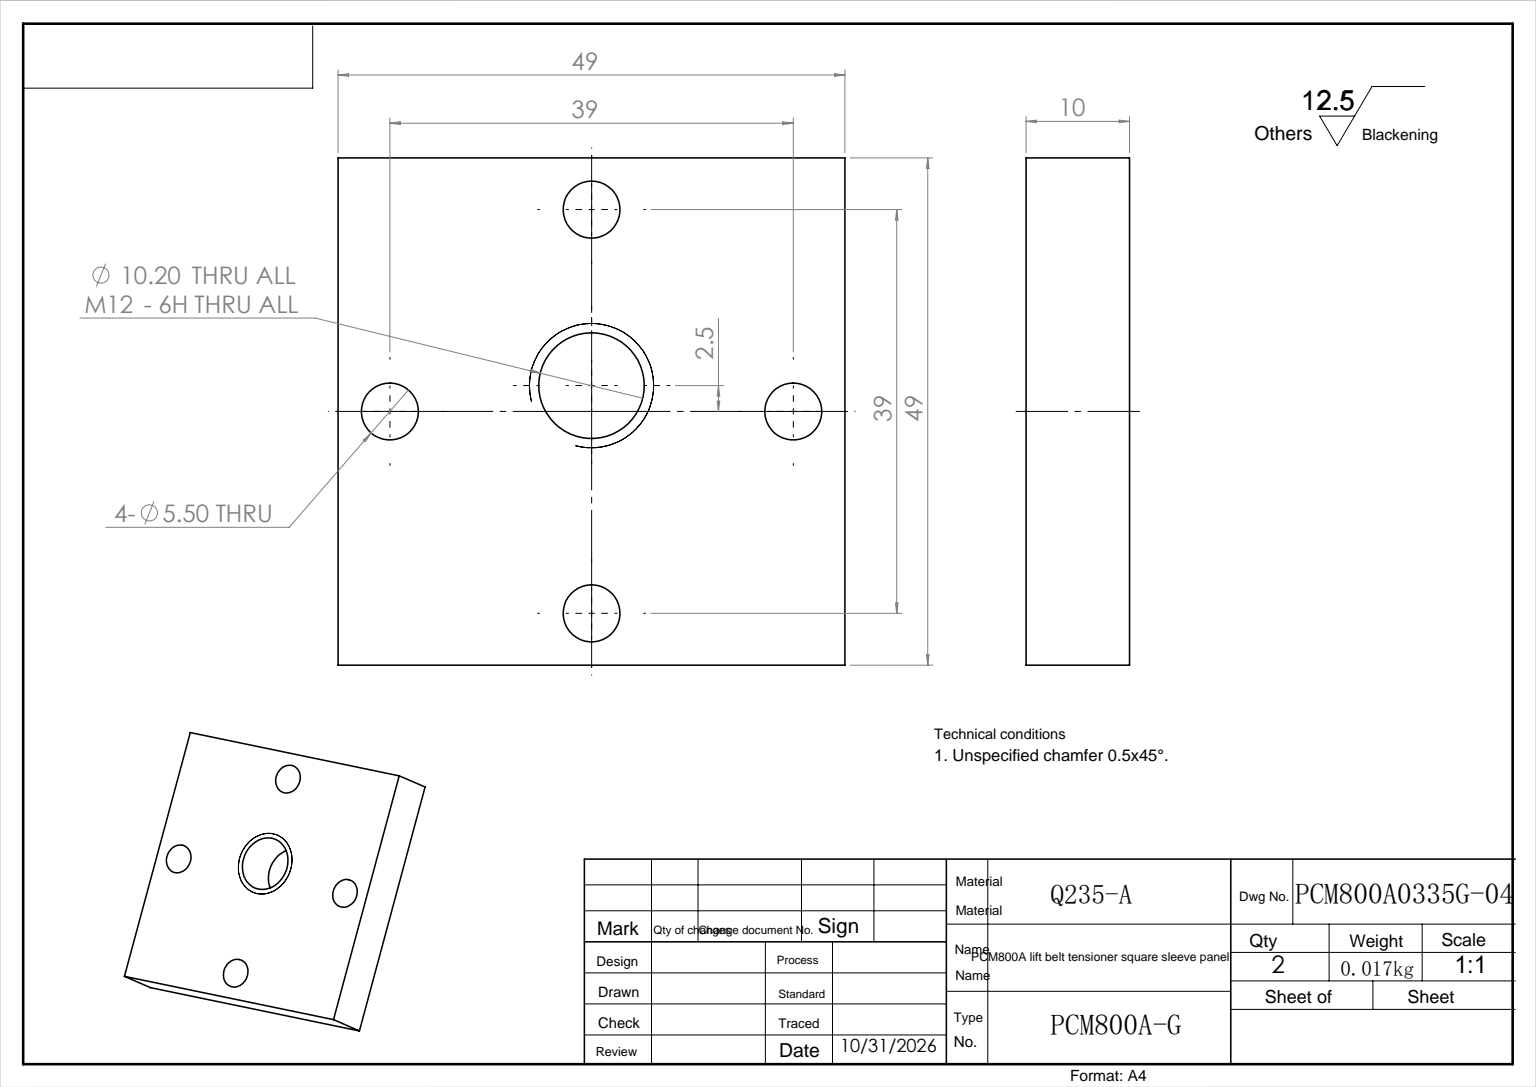
from build123d import *

# Parameters (mm, degrees)
SKETCH_1_W          = 49
SKETCH_1_H          = 49
EXTRUDE_1_DEPTH     = 10
SKETCH_2_R          = 2.75
CUT_EXTRUDE_1_DEPTH = 71.014284257
HOLE_WIZARD_M12_1_D = 10.2


with BuildPart() as part:
    # 草图1 → 拉伸1 (new body)
    with BuildSketch(Plane(origin=(0, 0, 0), x_dir=(1, 0, 0), z_dir=(0, 1, 0))):
        with Locations((24.5, 24.5)):
            Rectangle(SKETCH_1_W, SKETCH_1_H)
    extrude(amount=EXTRUDE_1_DEPTH)

    # 草图2 → 切除-拉伸1 (cut, through all)
    with BuildSketch(Plane(origin=(0, 10, 0), x_dir=(-1, 0, 0), z_dir=(0, 1, 0))):
        with Locations(Location((-24.5, -5, 0), (0, 0, 90))):
            Circle(SKETCH_2_R)
        with Locations(Location((-44, -24.5, 0), (0, 0, 90))):
            Circle(SKETCH_2_R)
        with Locations(Location((-24.5, -44, 0), (0, 0, 90))):
            Circle(SKETCH_2_R)
        with Locations(Location((-5, -24.5, 0), (0, 0, 90))):
            Circle(SKETCH_2_R)
    extrude(amount=-CUT_EXTRUDE_1_DEPTH, mode=Mode.SUBTRACT)

    # M12 螺纹孔1 (through all)
    with Locations(Plane(origin=(24.5, 10, -22), x_dir=(0, 0, 1), z_dir=(0, 1, 0))):
        with Locations((0, 0)):
            Hole(HOLE_WIZARD_M12_1_D / 2)


solid = part.part
